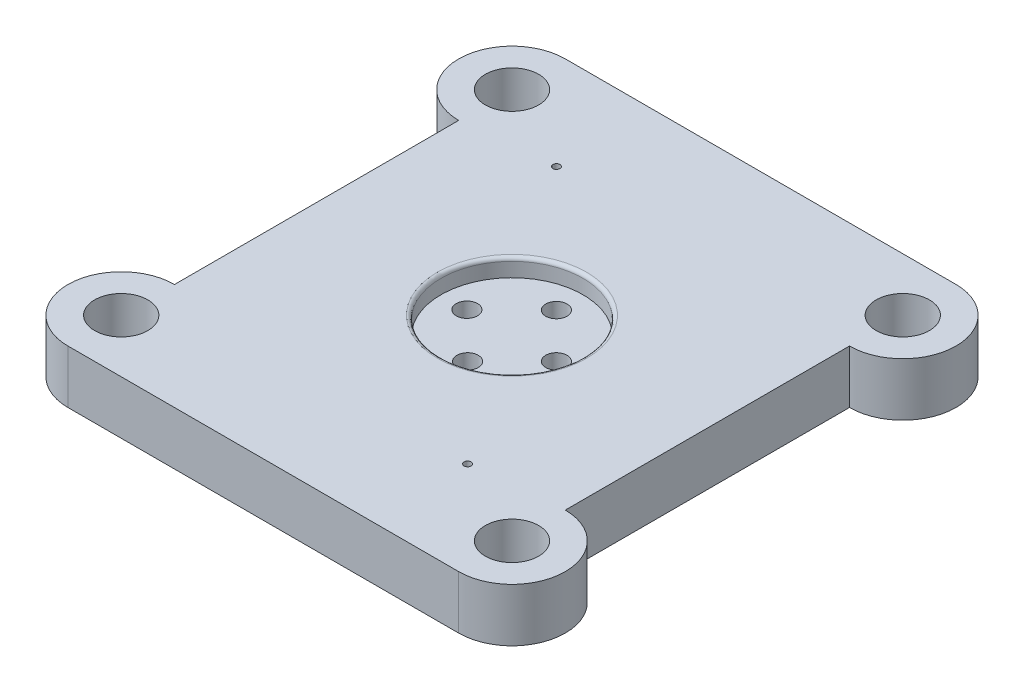
from build123d import *

# Parameters (mm, degrees)
SKETCH1_R                                        = 15
BOSS_EXTRUDE1_DEPTH                              = 30
CBORE_FOR_M8_PAN_HEAD_MACHINE_SCREW1_D           = 9
CBORE_FOR_M8_PAN_HEAD_MACHINE_SCREW1_CBORE_D     = 18
CBORE_FOR_M8_PAN_HEAD_MACHINE_SCREW1_CBORE_DEPTH = 6
SKETCH_1_R                                       = 2
CUT_EXTRUDE1_DEPTH                               = 201.249843945
SKETCH_3_R                                       = 5
CUT_EXTRUDE3_DEPTH                               = 20
SKETCH_4_R                                       = 40
CUT_EXTRUDE4_DEPTH                               = 10
FILLET1_R                                        = 2
SKETCH5_R                                        = 6
CUT_EXTRUDE7_DEPTH                               = 15


with BuildPart() as part:
    # Sketch1 → Boss-Extrude1 (new body)
    with BuildSketch(Plane(origin=(0, 0, 0), x_dir=(1, 0, 0), z_dir=(0, 1, 0))):
        with BuildLine():
            Line((-110, -140), (80, -140))
            Line((80, -140), (80, 140))
            Line((80, 140), (-110, 140))
            ThreePointArc((-110, 140), (-140, 110), (-110, 80))
            Line((-110, 80), (-110, -80))
            ThreePointArc((-110, -80), (-140, -110), (-110, -140))
        make_face()
        with Locations(Location((-110, 110, 0), (0, 0, 270))):
            Circle(SKETCH1_R, mode=Mode.SUBTRACT)
        with Locations(Location((-110, -110, 0), (0, 0, 270))):
            Circle(SKETCH1_R, mode=Mode.SUBTRACT)
    boss_extrude1 = extrude(amount=BOSS_EXTRUDE1_DEPTH)

    # CBORE for M8 Pan Head Machine Screw1 (through all)
    with Locations(Plane(origin=(0, 30, 0), x_dir=(1, 0, 0), z_dir=(0, 1, 0))):
        with Locations((60, 120), (-60, 120), (-60, -120), (60, -120)):
            CounterBoreHole(CBORE_FOR_M8_PAN_HEAD_MACHINE_SCREW1_D / 2, CBORE_FOR_M8_PAN_HEAD_MACHINE_SCREW1_CBORE_D / 2, CBORE_FOR_M8_PAN_HEAD_MACHINE_SCREW1_CBORE_DEPTH)

    # Mirror1: Boss-Extrude1 across plane
    add(boss_extrude1.mirror(Plane(origin=(0, 0, 0), x_dir=(0, 0, 1), z_dir=(1, 0, 0))))

    # 草图1 → Cut-Extrude1 (cut, through all)
    with BuildSketch(Plane(origin=(0, 30, 0), x_dir=(1, 0, 0), z_dir=(0, 1, 0))):
        with Locations(Location((-60, 85, 0), (0, 0, 270))):
            Circle(SKETCH_1_R)
        with Locations(Location((60, -85, 0), (0, 0, 270))):
            Circle(SKETCH_1_R)
    extrude(amount=-CUT_EXTRUDE1_DEPTH, mode=Mode.SUBTRACT)

    # 草图3 → Cut-Extrude3 (cut)
    with BuildSketch(Plane.XZ):
        with Locations(Location((-60, 120, 0), (0, 0, 270))):
            Circle(SKETCH_3_R)
        with Locations(Location((60, 120, 0), (0, 0, 90))):
            Circle(SKETCH_3_R)
        with Locations(Location((60, -120, 0), (0, 0, 270))):
            Circle(SKETCH_3_R)
        with Locations(Location((-60, -120, 0), (0, 0, 90))):
            Circle(SKETCH_3_R)
    extrude(amount=-CUT_EXTRUDE3_DEPTH, mode=Mode.SUBTRACT)

    # 草图4 → Cut-Extrude4 (cut)
    with BuildSketch(Plane(origin=(0, 30, 0), x_dir=(1, 0, 0), z_dir=(0, 1, 0))):
        with Locations(Location((0, 0, 0), (0, 0, 270))):
            Circle(SKETCH_4_R)
    extrude(amount=-CUT_EXTRUDE4_DEPTH, mode=Mode.SUBTRACT)

    # Fillet1
    fillet1_edges = [part.edges().sort_by_distance(p)[0] for p in [
        (0, 30, -40),
    ]]
    fillet(fillet1_edges, radius=FILLET1_R)

    # Sketch5 → Cut-Extrude7 (cut)
    with BuildSketch(Plane(origin=(0, 20, 0), x_dir=(1, 0, 0), z_dir=(0, 1, 0))):
        with Locations(Location((0, 25, 0), (0, 0, 270))):
            Circle(SKETCH5_R)
        with Locations(Location((-25.4, 0, 0), (0, 0, 270))):
            Circle(SKETCH5_R)
        with Locations(Location((25, 0, 0), (0, 0, 270))):
            Circle(SKETCH5_R)
        with Locations(Location((0, -25, 0), (0, 0, 270))):
            Circle(SKETCH5_R)
    extrude(amount=-CUT_EXTRUDE7_DEPTH, mode=Mode.SUBTRACT)


solid = part.part
